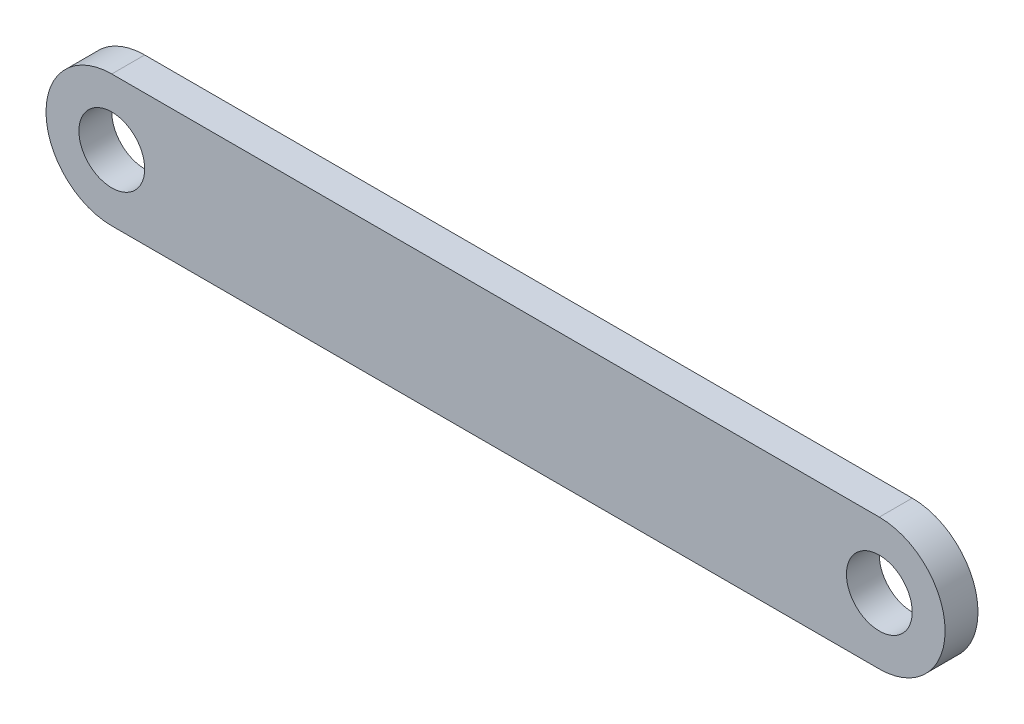
from build123d import *

# Parameters (mm, degrees)
SKETCH1_R           = 3
BOSS_EXTRUDE1_DEPTH = 3


with BuildPart() as part:
    # Sketch1 → Boss-Extrude1 (new body)
    with BuildSketch(Plane.XY):
        with BuildLine():
            Line((0, 6), (70, 6))
            ThreePointArc((70, 6), (76, 0), (70, -6))
            Line((70, -6), (0, -6))
            ThreePointArc((0, -6), (-6, 0), (0, 6))
        make_face()
        Circle(SKETCH1_R, mode=Mode.SUBTRACT)
        with Locations((70, 0)):
            Circle(SKETCH1_R, mode=Mode.SUBTRACT)
    extrude(amount=BOSS_EXTRUDE1_DEPTH)


solid = part.part
